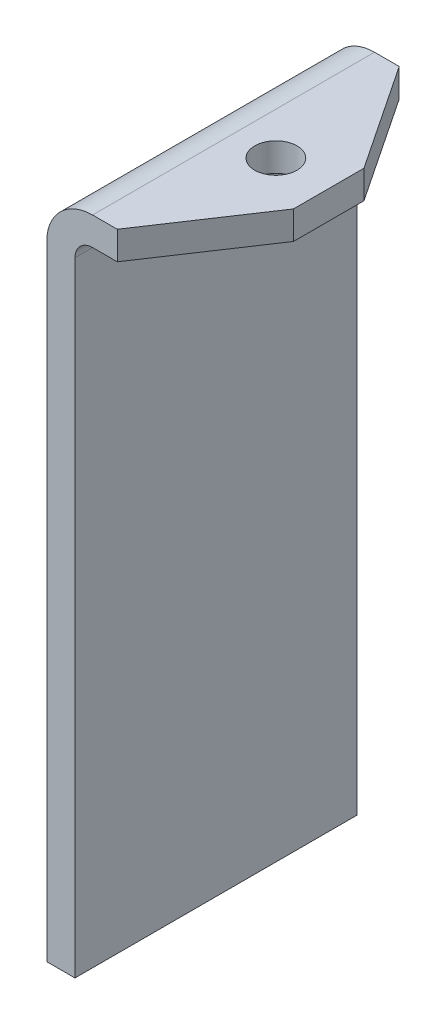
from build123d import *

# Parameters (mm, degrees)
BOSS_EXTRUDE1_DEPTH = 80
SKETCH2_R           = 6
CUT_EXTRUDE1_DEPTH  = 12


with BuildPart() as part:
    # Sketch1 → Boss-Extrude1 (new body)
    with BuildSketch(Plane.XY):
        with BuildLine():
            Line((0, 0), (-27, 0))
            ThreePointArc((-27, 0), (-36.192388155, -3.807611845), (-40, -13))
            Line((-40, -13), (-40, -190))
            Line((-40, -190), (-32, -190))
            Line((-32, -190), (-32, -13))
            ThreePointArc((-32, -13), (-30.535533906, -9.464466094), (-27, -8))
            Line((-27, -8), (0, -8))
            Line((0, -8), (0, 0))
        make_face()
    extrude(amount=BOSS_EXTRUDE1_DEPTH)

    # Sketch2 → Cut-Extrude1 (cut)
    with BuildSketch(Plane(origin=(0, 0, 0), x_dir=(1, 0, 0), z_dir=(0, 1, 0))):
        with Locations(Location((-15, -40, 0), (0, 0, 270))):
            Circle(SKETCH2_R)
        Polygon((-20, 0), (0, -30), (0, 0), align=None)
        Polygon((0, -50), (0, -80), (-20, -80), align=None)
    extrude(amount=-CUT_EXTRUDE1_DEPTH, mode=Mode.SUBTRACT)


solid = part.part
